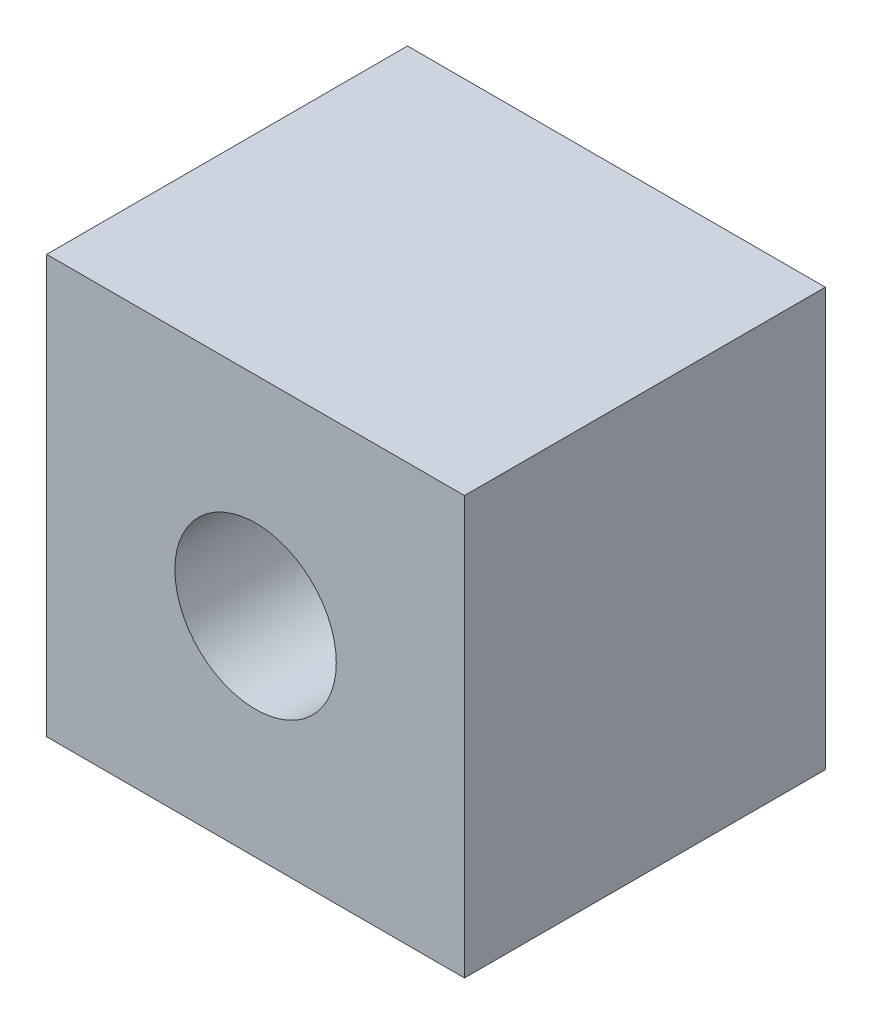
from build123d import *

# Parameters (mm, degrees)
SKETCH1_W              = 22
SKETCH1_H              = 22
SKETCH1_R              = 4
BOSS_EXTRUDE1_DEPTH    = 19
M10_TAPPED_HOLE2_D     = 8.5
M10_TAPPED_HOLE2_DEPTH = 27.5
M10_TAPPED_HOLE2_TIP   = 2.553657631


with BuildPart() as part:
    # Sketch1 → Boss-Extrude1 (new body)
    with BuildSketch(Plane.XY):
        with Locations((866.772265526, 975.162817643)):
            Rectangle(SKETCH1_W, SKETCH1_H)
        with Locations((866.772265526, 975.162817643)):
            Circle(SKETCH1_R, mode=Mode.SUBTRACT)
    extrude(amount=BOSS_EXTRUDE1_DEPTH)

    # M10 Tapped Hole2
    with Locations(Plane(origin=(866.772265526, 975.162817643, 19), x_dir=(1, 0, 0), z_dir=(0, 0, 1))):
        with Locations((0, 0)):
            Hole(M10_TAPPED_HOLE2_D / 2, depth=M10_TAPPED_HOLE2_DEPTH)
            with Locations((0, 0, -(M10_TAPPED_HOLE2_DEPTH + M10_TAPPED_HOLE2_TIP / 2))):  # 118° drill point
                Cone(0, M10_TAPPED_HOLE2_D / 2, M10_TAPPED_HOLE2_TIP, mode=Mode.SUBTRACT)


solid = part.part
